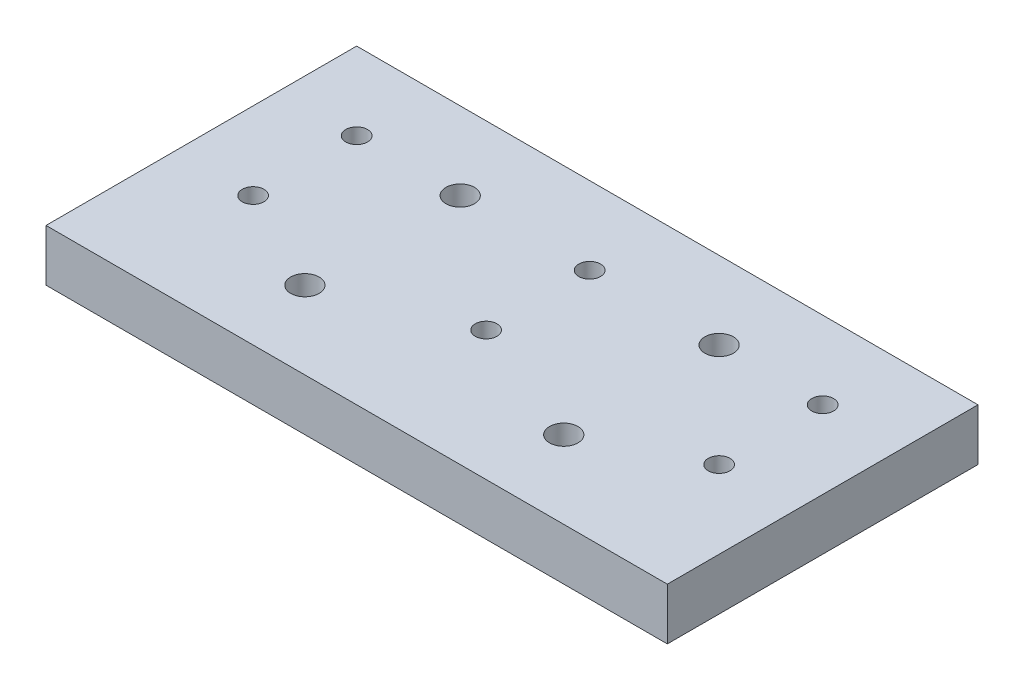
from build123d import *

# Parameters (mm, degrees)
SKETCH_1_W                                         = 120
SKETCH_1_H                                         = 60
BOSS_EXTRUDE_1_DEPTH                               = 10
M5_SOCKET_HEAD_CAP_SCREW_COUNTERBORE_1_D           = 5.5
M5_SOCKET_HEAD_CAP_SCREW_COUNTERBORE_1_CBORE_D     = 10
M5_SOCKET_HEAD_CAP_SCREW_COUNTERBORE_1_CBORE_DEPTH = 5
LINEAR_PATTERN_1_COUNT                             = 2
LINEAR_PATTERN_1_PITCH                             = 50
LINEAR_PATTERN_1_COUNT_DIR2                        = 2
LINEAR_PATTERN_1_PITCH_DIR2                        = 30
M5_TAPPED_HOLE_1_D                                 = 4.2
LINEAR_PATTERN_2_COUNT                             = 2
LINEAR_PATTERN_2_PITCH                             = 20
LINEAR_PATTERN_2_COUNT_DIR2                        = 3
LINEAR_PATTERN_2_PITCH_DIR2                        = 45


with BuildPart() as part:
    # Sketch 1 → Boss-Extrude 1 (new body)
    with BuildSketch(Plane(origin=(0, 0, 0), x_dir=(1, 0, 0), z_dir=(0, 1, 0))):
        Rectangle(SKETCH_1_W, SKETCH_1_H)
    extrude(amount=BOSS_EXTRUDE_1_DEPTH)

    # M5 Socket Head Cap Screw Counterbore 1 (through all)
    with Locations(Plane.XZ):
        with Locations((-25, 15)):
            m5_socket_head_cap_screw_counterbore_1 = CounterBoreHole(M5_SOCKET_HEAD_CAP_SCREW_COUNTERBORE_1_D / 2, M5_SOCKET_HEAD_CAP_SCREW_COUNTERBORE_1_CBORE_D / 2, M5_SOCKET_HEAD_CAP_SCREW_COUNTERBORE_1_CBORE_DEPTH)

    # Linear Pattern 1: M5 Socket Head Cap Screw Counterbore 1 2 × 2
    with Locations(*[(i * LINEAR_PATTERN_1_PITCH, 0, -j * LINEAR_PATTERN_1_PITCH_DIR2) for i in range(LINEAR_PATTERN_1_COUNT) for j in range(LINEAR_PATTERN_1_COUNT_DIR2) if (i, j) != (0, 0)]):
        add(m5_socket_head_cap_screw_counterbore_1, mode=Mode.SUBTRACT)

    # M5 Tapped Hole 1 (through all)
    with Locations(Plane.XZ):
        with Locations((-45, 5)):
            m5_tapped_hole_1 = Hole(M5_TAPPED_HOLE_1_D / 2)

    # Linear Pattern 2: M5 Tapped Hole 1 2 × 3
    with Locations(*[(j * LINEAR_PATTERN_2_PITCH_DIR2, 0, -i * LINEAR_PATTERN_2_PITCH) for i in range(LINEAR_PATTERN_2_COUNT) for j in range(LINEAR_PATTERN_2_COUNT_DIR2) if (i, j) != (0, 0)]):
        add(m5_tapped_hole_1, mode=Mode.SUBTRACT)


solid = part.part
